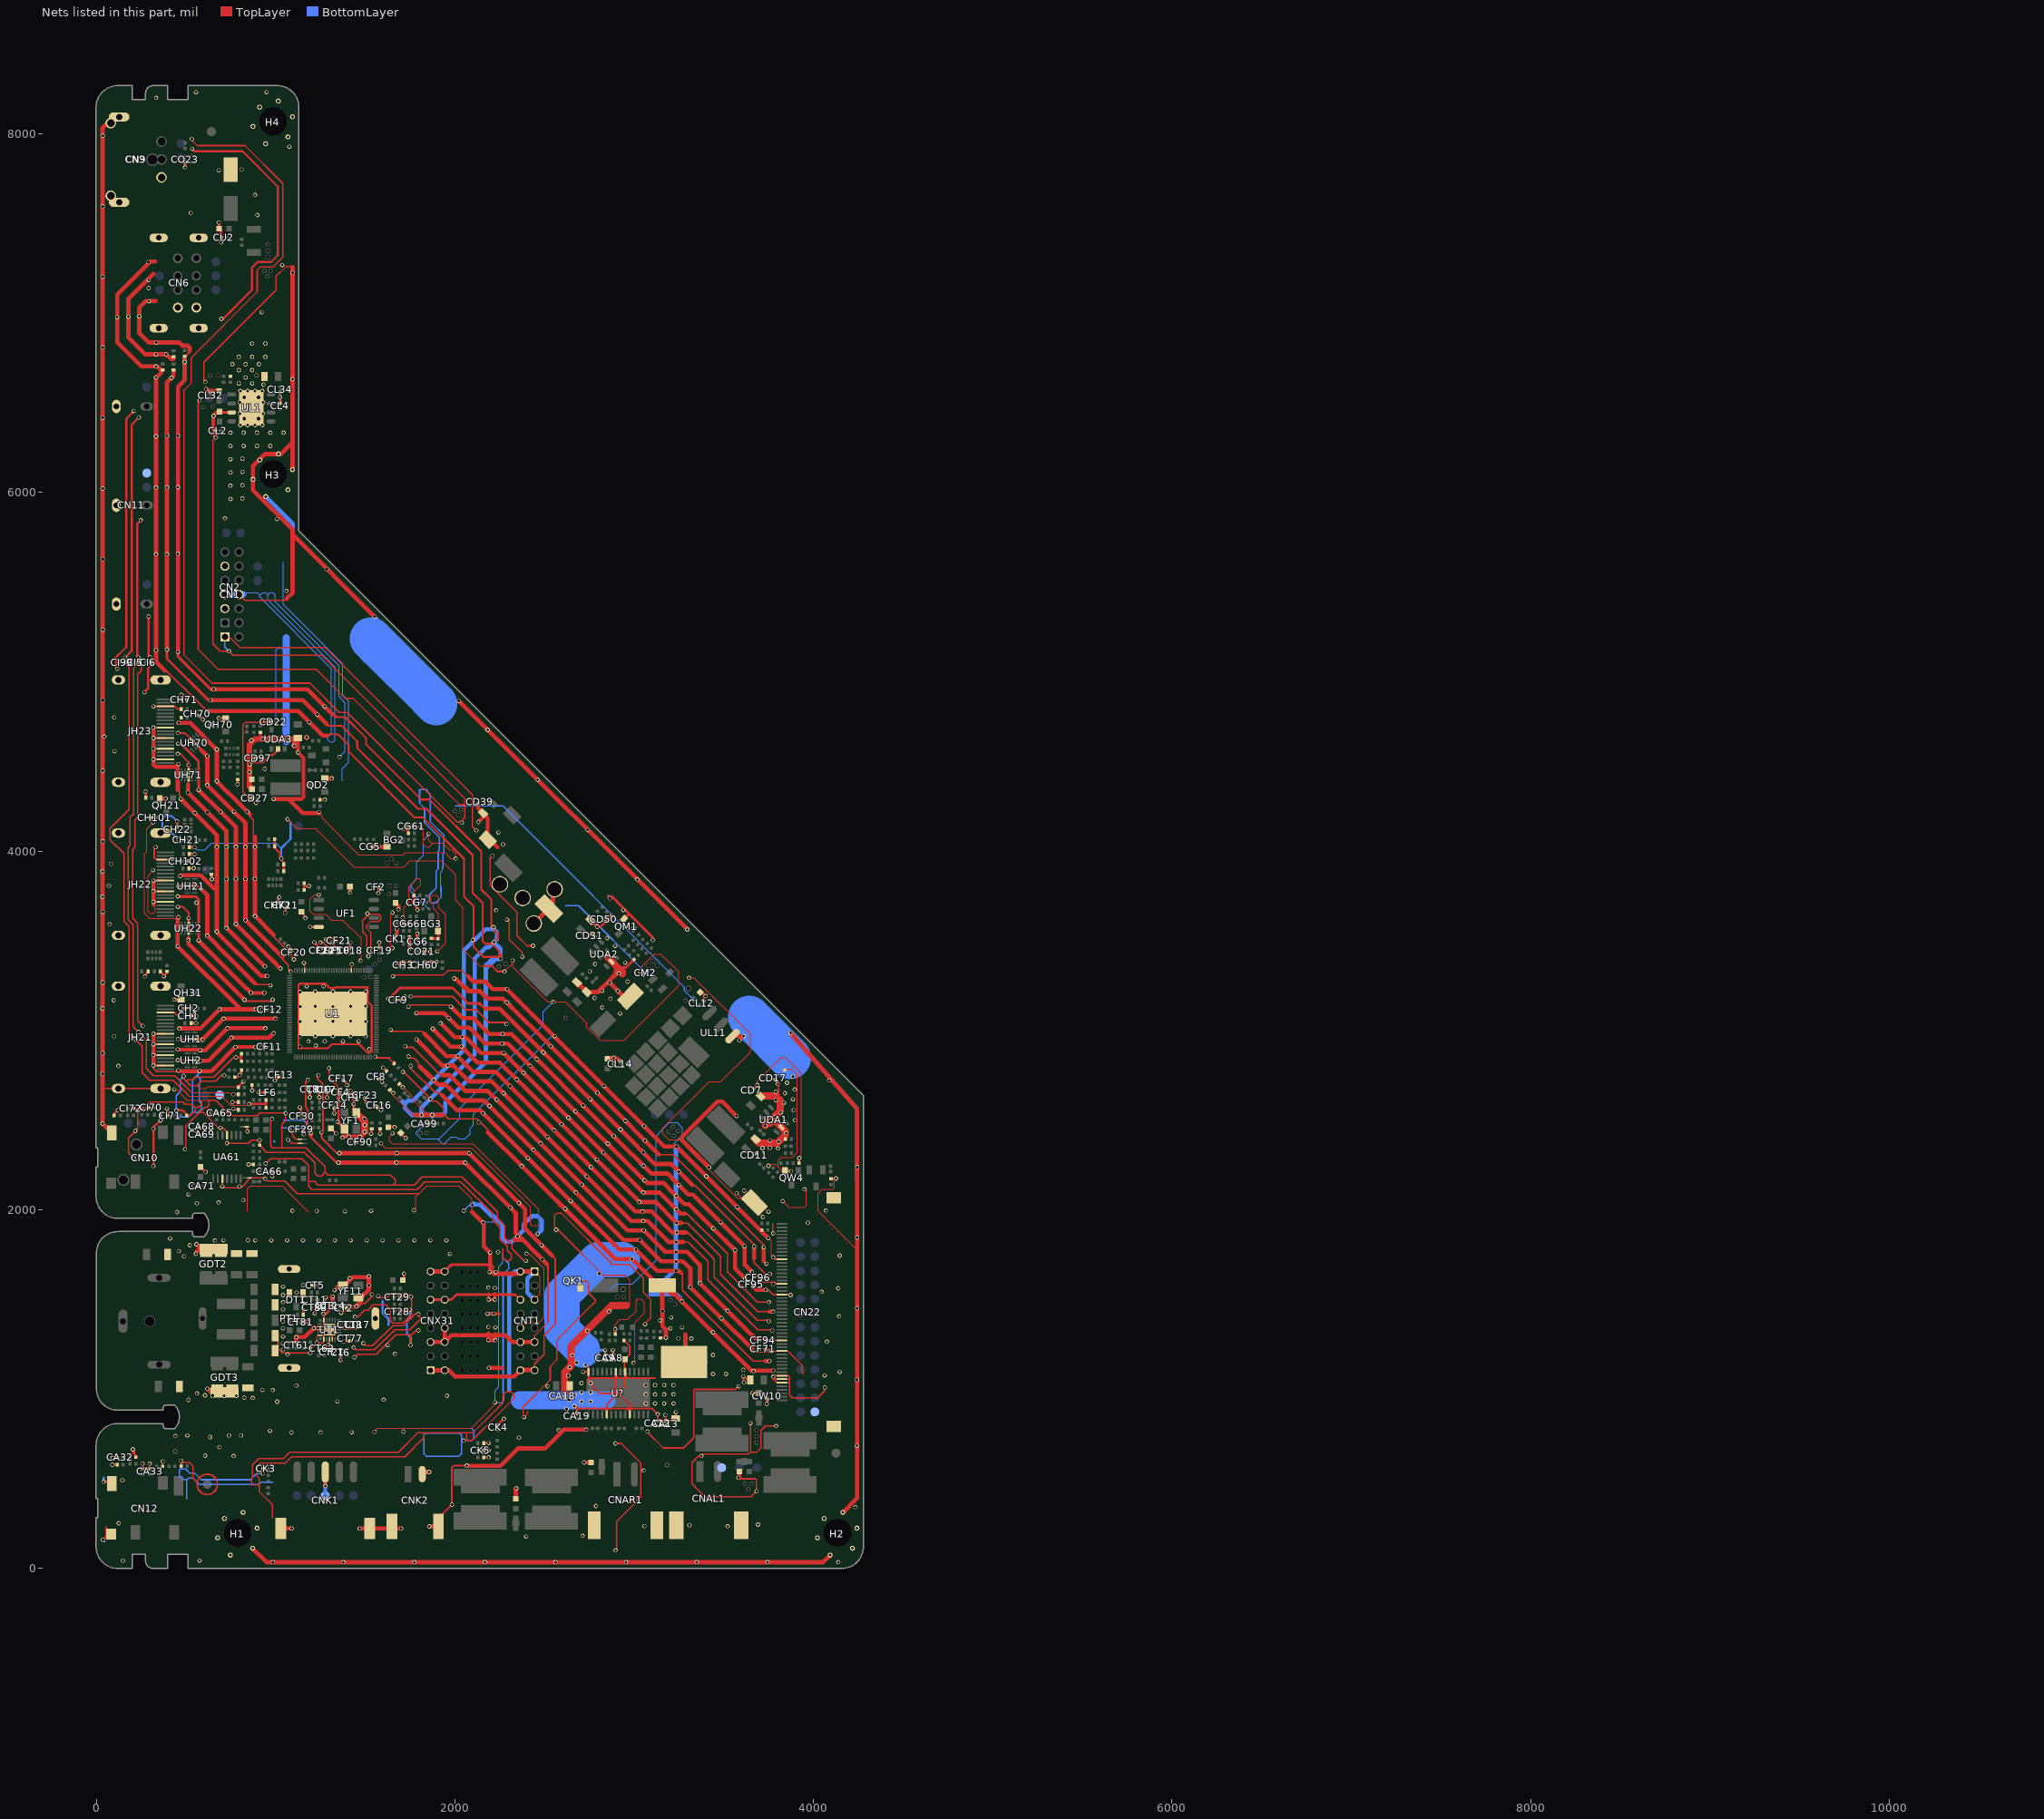
[diagram p0: the nets of this part, all layers, seen from the top]
# Altium PCB MISC105950.PcbDoc (part 8 of 15)
Units mil, origin at the board's own origin, x right, y up, seen from the top; angles counter-clockwise.
Board outline 4280.62 x 8272.76 mil, 2 copper layers (TopLayer, BottomLayer), stack 61.855 mil thick; 541 components, 268 nets, 2324 pads, 1157 vias.

## Via types
v1: diameter 23.62, hole 15.75, TopLayer to BottomLayer, tented both sides, 1087 vias
v2: diameter 23.62, hole 15.75, TopLayer to BottomLayer, 51 vias
v3: diameter 27.56, hole 19.68, TopLayer to BottomLayer, 15 vias
v4: diameter 31.5, hole 19.68, TopLayer to BottomLayer, tented both sides, 4 vias

## Nets (pads, with @x,y where several pads share a name; then routed paths per layer and width w, separated by ;. In a path a pad name is that pad's centre, name@x,y a point inside that pad or via, vN(x,y) a via of type N, cw(c..) or ccw(c..) an arc to the next point about the centre after c; other vN are vias at no path point) (continued)
GND: (continued)
  TopLayer w8: 41.8,2675.2 JH21.23@121.65,2675.2 JH21.22@356.3,2675.2 ; DA53.A@256.5,555.73 v2(256.5,582.5) ; CA33.2@297,555.24 v2(297,582) ; v2(369,595) 369.23,594.77 RA56.1@369.23,567 ; v1(432,2671) 443.41,2671 501.41,2613 ; DA51.A@471.27,565.23 DA51.A@471.27,568.5 471.27,597.27 v2(471.5,597.5) ; v2@471.27,588 471.59,588.33 495.5,588.33 ; v1@486,2743 v1(486,2743.5) ; 488,5163.35 488,5181.5 ; 491.09,588.33 495.5,588.33 ; v1(532,7972.38) 532,7963.5 534.61,7960.89 536.3,7960.89 561.69,7935.5 828.01,7935.5 1039.5,7724.01 1039.5,7312.78 984.72,7258 979.23,7258 979.12,7258.11 961.88,7258.11 961.77,7258 945.23,7258 ; 559.5,478.5 538,500 538,568 517.67,588.33 495.5,588.33 ; v1(574,6514) 567,6507 567,6486.5 ; v1@575,6514 575,6513 567,6505 567,6486.5 ; 575.25,2542.07 593.65,2542.07 679.71,2456 v1(691,2456) ; v1(606,6617.5) 599,6624.5 599,6726.95 1001.5,7129.45 1001.5,7206.88 1055,7260.38 1090.97,7260.38 ; v1(610.5,6578) 628.5,6560 CL32.2@635.43,6560 642.5,6567.07 CL31.2@683.93,6567.07 ; 648.5,6356.77 CL2.1@658,6347.27 ; 658.95,5145.42 649,5155.37 ; v1(665.5,6307) 649,6290.5 649,5155.37 ; 675,4936.5 692,4936.5 ; 712.09,5014.5 741.5,5014.5 ; CN1.1@715.6,5195.1 739.9,5195.1 799.5,5135.5 1275.66,5135.5 2097.5,4313.66 2097.5,4136 v1@2121.27,4112.23 ; CN2.6@794.34,5431.32 826.17,5399.5 1048,5399.5 1068.5,5420 ; 816.65,4705.7 829.64,4718.69 930.69,4718.69 v1(941,4729) ; 816.65,4705.9 816.65,4330.04 851.19,4295.5 CD27.1@865.43,4295.5 ; 816.65,4774.65 822.5,4780.5 ; 906.5,462.5 877.5,462.5 864.69,475.31 864.69,482 864.69,496.12 869.5,500.93 869.5,575.48 904.73,610.71 933,610.71 1042.33,610.71 1069.81,638.19 1078,646.38 1683.76,646.38 1792.73,755.35 2066,755.35 ; CK3.2@928.26,554.5 928.26,526.74 v2(928.5,526.5) ; 945.22,7258.01 914.01,7258.01 896,7240 896,7120.12 528.5,6752.62 528.5,6612 488,6571.5 488,5181.5 ; 980.5,279.5 980.5,335.5 ; 980.5,319 980.5,353 906.5,427 906.5,501.5 895.5,512.5 895.5,564.71 915.5,584.71 953,584.71 1053.1,584.71 1078.69,610.31 ; CT41.1@1012.06,1223.5 1035.56,1200 v1(1192.5,1200) ; 1071.69,603.31 1078.69,610.31 ; v1(1153,1442) v1@1153.23,1441.77 ; v1(1157,3377) 1160.04,3373.96 1160.04,3348 ; U1.124@1160.04,3334.04 1160.04,3348 ; 1160.04,3364.2 1160.04,3348 ; v1@1160.04,3367.05 1160.04,3348 ; 1172,5014.5 1163.5,5014.5 ; v1@1184.19,1191.68 v1(1192.5,1200) ; v1@1220.42,1330 v1(1212.89,1337.53) v1@1221.1,1345.75 ; 1229,1281.53 v1(1229,1256.5) ; 1260.78,1256.5 v1(1229,1256.5) ; UT1.EPAD@1283.75,1345.75 UT1.EPAD@1299.5,1330 ; v2(1294.25,1244.78) 1294.25,1240.97 CT21.1@1313,1222.23 ; U1.105@1421.85,3334.04 1421.85,3366.85 v1(1423.5,3368.5) ; v1@1470.98,3387.23 v1(1472.12,3388.38) ; v1(1511,3651) 1514.69,3647.31 1529,3647.31 ; v1(1516,3413.5) 1514.26,3411.76 1507.81,3418.21 1507.81,3526.4 1485.06,3549.15 1485.06,3612.12 1520.25,3647.31 1529,3647.31 ; v1(1539,3445.5) 1530.81,3453.69 1530.81,3545.13 1508.06,3567.88 1508.06,3585.12 1528.63,3605.69 1572.92,3605.69 1585.11,3617.88 1585.11,3635.12 1572.92,3647.31 1529,3647.31 ; v1(1653.25,3301.19) v1@1653.25,3307.81 ; v1@1654.44,3309 1654.44,3308.9 1717.5,3308.9 ; 1690.14,3309 1690.24,3308.9 1717.5,3308.9 ; 1831.5,755.35 1825.14,748.98 1825.14,726.21 1719.31,620.38 1088.77,620.38 1078.69,610.31 ; 1909.5,2527.31 1917.5,2519.31 ; v1@2038,4157.5 v1(2038,4158.5) ; v1(2048.58,711.19) 2075.38,711.19 ; 2054.5,4258.5 2024.5,4258.5 1948.18,4334.82 1430.13,4852.87 1384.92,4852.87 1223.29,5014.5 1163.5,5014.5 ; 2089.95,3284.05 2040,3334 1961.3,3334 1936.3,3309 1728.86,3309 1728.76,3308.9 1717.5,3308.9 ; CD96.1@2140.67,4213.05 2174.29,4179.42 ; v1(2208,3973.5) 2195.64,3961.14 2195.64,3808.36 2345.5,3658.5 2345.5,3527.85 2401.85,3471.5 v1(2434.5,3471.5) ; 2220.5,874.74 2207.63,861.87 ; v1(2229,3669.5) v1@2239,3669.5 ; 2256.69,910.93 2266.81,921.05 ; 2262.31,879.78 2244.52,861.98 ; 2266.81,930.69 2266.81,963.81 ; v1(2288.5,3617.5) 2288.5,3626 2290,3627.5 2302,3615.5 2302,3506.5 2374.87,3433.63 v1(2374.87,3410.13) ; v1@2379.9,840.7 2379.9,898.37 2530.86,1049.34 2530.86,1124.63 2566.86,1160.63 2566.86,1270.96 2740.2,1444.3 ; v1(2385,841) 2404,860 2404,873 ; 2556.19,1968.12 2568.38,1980.31 ; v1(2563.62,1886.98) 2574.67,1886.98 2600.83,1860.83 ; v1(2699,1600) 2735.5,1600 2744.5,1591 2744.5,1534.5 2782.4,1496.6 2782.4,1486.5 2740.2,1444.3 ; 2745.45,1449.55 2740.2,1444.3 ; 2750.85,1454.94 2740.2,1444.3 ; v1(2894.5,695) 2926.38,695 3035.5,585.88 3035.5,393.5 2902.5,260.5 2902.5,106 v1(2895,98.5) ; 2948.67,1632 2829.65,1632 2600.83,1860.83 ; v1(3060,1360) 3058,1362 3058,1363 3091.45,1396.45 3091.45,1497.78 3050,1539.24 3050,1616.93 2973.93,1693 2878.9,1693 2591.59,1980.31 2568.38,1980.31 ; v1@3071.5,759 3160.83,669.67 3196,669.67 ; RA1.2@3145.5,1284.27 v1(3176.23,1284.27) ; 3165.33,669.67 3196,669.67 ; 3301.5,697 3274.17,669.67 3196,669.67 ; 3337.6,603.5 3359.1,625 ; v1(3374.5,625) 3359.1,625 ; 3386.5,635.5 3376,625 3376,631 3380.5,635.5 3636.66,635.5 ; 3468.5,635.5 3636.66,635.5 ; v1(3580.19,503.94) 3586.63,497.5 3676.5,497.5 3681.5,492.5 v1(3681.5,428) 3650.5,397 3395,397 3322,470 3322,587.9 3359.1,625 ; 3647.5,644.5 v1(3647.5,808) ; v1(3763.2,1210.82) 3782,1210.82 ; v1@3768.62,1210.82 3782,1210.82 ; 3772.5,1923.5 3772.5,1869.76 v1(3775.11,1867.15) ; v1@3781.5,2617.5 3805.5,2641.5 3805.5,2702.5 CD17.2@3785.33,2722.67 3785.33,2715.17 v1(3800.5,2700) ; v1(3791.5,792) 3732.31,792 3707,766.69 3707,670.12 3681.86,644.98 3646.14,644.98 3636.66,635.5 ; 3945,1085 3934,1096 3934,1132.65 3863.02,1203.63 3862.69,1203.63 3855.51,1210.82 CN22.15@3823.43,1210.82 3782,1210.82 ; 488,5181.5 488,5093.29 644.79,4936.5 692,4936.5 ; 567,6486.5 567,5124.6 677.1,5014.5 741.5,5014.5 ; 649,5155.37 689.98,5114.39 v1(739.14,5114.39) 761.03,5092.5 1255.59,5092.5 2054.5,4293.59 2054.5,4186 2030.5,4162 2010.69,4162 1398.69,4774 1353,4774 1190.5,4936.5 692,4936.5 ; 741.5,5014.5 1163.5,5014.5 ; v1(1192.5,1200) LT4.1@1192.5,1226.77 1199.27,1226.77 v1(1229,1256.5) ; 2066,755.35 2101.11,755.35 2207.63,861.87 ; 2066,755.35 2063.19,752.54 2063.19,723.38 2075.38,711.19 ; 2075.38,711.19 2093.72,711.19 2244.52,861.98 ; 2207.63,861.87 2266.81,921.05 ; 2244.52,861.98 2330.52,947.98 2330.52,964.98 2313.5,982 2285,982 2266.81,963.81 ; 2266.81,921.05 2266.81,963.81 ; 2568.38,1980.31 2555.81,1967.74 2555.81,1905.84 2600.83,1860.83
  TopLayer w9: v1@3775.92,1733.23 3786.52,1722.63 CN22.41@3823.43,1722.63
  TopLayer w10: v1(317,2803) 317.15,2803.15 JH21.2@384.16,2803.15 ; v1(317,2862) 317.21,2862.21 JH21.5@384.16,2862.21 ; v1(317,2921.5) 317.24,2921.26 JH21.8@384.16,2921.26 ; v1(317,2980.5) 317.18,2980.32 JH21.11@384.16,2980.32 ; v1@317,3716.33 v1@317.21,3716.54 ; v1(317,3716.5) 317.04,3716.54 JH22.5@384.16,3716.54 v1@317.94,3716.54 ; v1(317,3775.83) 317.24,3775.59 317.94,3775.59 JH22.8@384.16,3775.59 ; v1(317,3834.83) 317.18,3834.65 JH22.11@384.16,3834.65 ; v1(317,4511.66) 317.15,4511.81 JH23.2@384.16,4511.81 ; v1(317,4570.66) 317.21,4570.87 JH23.5@384.16,4570.87 ; v1(317,4630.16) 317.24,4629.92 JH23.8@384.16,4629.92 ; v1(317,4689.16) 317.18,4688.98 JH23.11@384.16,4688.98 ; v1(317,4807) 317.09,4807.09 JH23.17@384.16,4807.09 436,4807.09 451.59,4791.5 DH72.A@472.77,4791.5 ; v1(330,4021.78) 321,4012.78 321,3964.5 332.74,3952.76 JH22.17@384.16,3952.76 ; 332,5060.49 335.54,5060.49 615.53,4780.5 v1(622.51,4780.5) ; JH21.17@384.16,3098.43 435.07,3098.43 v1(462.5,3071) ; v1@451.62,3686.71 451.62,3686.78 v1(452.95,3688.11) 482.39,3688.11 512.98,3657.52 v1@512.98,3613.5 ; v1@451.62,4541.04 451.62,4541.12 v1(452.95,4542.44) 466.06,4542.44 512.98,4495.52 UH71.GND@512.98,4444.3 ; v1(452.95,2833.78) 451.62,2832.45 451.62,2832.38 UH2.GND@547.47,2832.38 ; v1(454.5,2950.5) 454.62,2950.38 524.5,2950.38 ; v1@454.62,4659.04 v1(454.5,4659.16) 492.54,4659.16 UH70.GND@532.22,4619.48 ; v1(455.71,3804.71) 522.5,3804.71 ; v1(469.09,3123.27) 469.36,3123 CH2.2@495.76,3123 ; UH21.GND@506.53,3804.71 522.5,3804.71 ; UH22.GND@512.98,3549.03 v1@512.98,3613.5 ; UH22.GND@512.98,3589.97 v1@512.98,3613.5 ; 544.93,4606.78 580.72,4570.99 ; UH1.GND@547.47,2950.38 524.5,2950.38 ; 575.11,2950.38 524.5,2950.38 ; v1@580.22,3791.06 566.57,3804.71 522.5,3804.71 ; v1@640,3840 DH4.A@640,3866.77 ; v1(643,2539.5) CA65.2@671.26,2539.5 ; v1(691,2456) 704.5,2456 727.18,2433.32 UA61.4@727.18,2414.61 ; v1(758,2598) 759,2599 DI2.A@790.27,2599 ; v1(763,2562) 768.5,2556.5 DI33.A@789.77,2556.5 ; v1(824.82,3170.5) 831.82,3163.5 975.65,3163.5 v1(982.47,3170.31) ; RA64.JP_2K@837.76,2461.54 841,2458.3 v1(841,2436.5) ; CT41.1@1012.06,1223.5 CT42.1@1012.06,1309.37 ; v1(1178,2723) 1168,2713 1168,2569.59 1176.5,2561.09 1176.5,2447 v1(1194.5,2429) ; 1194.5,2405.96 1338.96,2261.5 v1(1348.86,2261.5) ; v1(1237.22,2748.94) 1233.5,2745.22 1233.5,2729 1263.84,2698.66 1263.84,2440.62 1254.84,2431.62 v1(1254.84,2430.47) 1254.84,2400.77 1341.11,2314.5 1370.81,2314.5 v1@1360.91,2314.5 ; CT10.2@1241,2652.76 1241,2627.72 v1(1242.62,2626.09) ; 1268,1406.52 1295.84,1434.36 1295.84,1473.66 1289.77,1479.73 CT3.1@1276,1479.73 ; v1(1554.5,2852.5) 1561.5,2845.5 1602.5,2845.5 ; v1(1598.61,2791.69) 1598.61,2791.39 DU31.A@1617.73,2772.27 ; 1636.15,2845.5 1602.5,2845.5 ; DU33.A@1636.33,2668.17 1655.16,2649.34 v1(1655.22,2649.34) ; DU32.A@1660.67,2814.33 1629.5,2845.5 1602.5,2845.5 ; DU34.A@1688.83,2700.67 1707.29,2682.21 v1(1708.09,2682.21) ; v1(1721.5,2910.5) 1728.44,2903.56 1765.14,2903.56 1919.02,2749.68 1928.92,2749.68 ; v1(1753,3189) 1787,3189 ; v1@1761.5,3189 1787,3189 ; CNK2.4@1907.13,277.89 v1(1982.86,353.62) 1982.86,462.5 ; 1982.86,441.36 1982.86,462.5 ; 2038.05,3261 2043.52,3255.52 2039.98,3255.52 ; 2066.5,3307.5 2103,3271 ; 2078.71,575.71 2073,570 1992,570 1982.86,560.86 1982.86,462.5 ; v1@2292,3040 2289,3043 2191.19,3043 2120.51,3113.68 2059.89,3113.68 1984.57,3189 1787,3189 ; v1(2486.69,1721.55) 2486.69,1721.82 2473,1735.5 2473,1725.61 2519,1679.61 2519,1663.5 ; 2519,1374.42 2519,1663.5 ; 2519,1699.41 2519,1663.5 ; 2529.78,1753.68 2558,1725.46 2558,1362.5 ; v1(2636,937.5) 2636,937.73 CA18.1@2615.23,958.5 2639.53,982.8 CA2.1@2639.53,1017 ; 2672.98,889.93 3098.57,889.93 v1(3130.5,858) CA12.1@3130.5,823.23 3221.2,823.23 CA1.1@3231,833.03 v1(3231,869) ; CA19.1@2680,865.23 2680,899.5 ; v1(2714.5,1094.5) U?.14@2743.87,1094.5 ; v1(2727.87,1132.13) 2743.87,1116.14 U?.14@2743.87,1094.5 ; 2830.23,889.93 U?.19@2846.23,873.93 ; U?.19@2846.23,854.34 2846.23,910.44 2910.2,974.42 ; U?.19@2846.23,877.14 2859.02,889.93 ; 2884.61,1058.91 2897.41,1071.7 ; 2897.41,987.22 U?.8@2897.41,1094.5 ; U?.8@2897.41,1074.91 2913.41,1058.91 ; 2935.8,1058.91 2948.59,1071.7 U?.6@2948.59,1094.5 ; RA9.1@2942.77,1270 2942.95,1270 2972.75,1240.2 2972.75,1190.44 CA7.1@2957.61,1175.3 ; U?.6@2947,1096.09 CA7.1@2947,1164.69 ; 2958.18,889.93 U?.24@2974.18,873.93 ; 2964.59,1058.91 2948.59,1074.91 U?.6@2948.59,1094.5 ; U?.24@2974.18,854.34 2974.18,910.44 2910.2,974.42 ; U?.24@2974.18,877.14 2986.98,889.93 ; v1@3071.5,759 3071.5,759.5 v1(3073.5,761.5) ; 3116.09,1058.91 2757.46,1058.91 2743.87,1072.5 U?.14@2743.87,1094.5 ; CA13.1@3173,822.89 v1(3173,853.5) ; 3275.17,670.67 3331.86,727.36 3331.86,811 ; 3331.86,769.36 3331.86,811 ; v1@3583,1016 3564.29,997.29 3337.72,997.29 3331.86,991.43 3331.86,811 ; v1(3611.65,1035.18) 3608,1038.83 v1(3608,1069) 3612,1069 3632,1049 CW9.1@3647.47,1049 ; v1(3659,975) v1@3659.31,975.31 ; U?.14@2743.87,1094.5 2743.87,1037.13 2806.58,974.42 2910.2,974.42 ; 2910.2,974.42 2948.59,1012.81 U?.6@2948.59,1094.5
  TopLayer w11: 1255.88,4650.5 1347.54,4650.5 1406.5,4591.54 1406.5,4554.99 1774.49,4187 1820.53,4187 2050.5,3957.03 2050.5,3745.5 2103.15,3692.85 2103.15,3580 ; 1284.96,4707.69 1294.15,4698.5 1340.5,4698.5 ; 1312,4698.5 1340.5,4698.5 ; CF3.1@1413.81,3802 1414,3801.81 v1(1414,3768) ; CG7.1@1767.27,3714 CG7.1@1770,3716.73 ; v1(2099,3504) 2103.15,3508.15 2103.15,3580 ; 2165.42,3358.5 2206.17,3358.5 2236.67,3328 v1(2275,3328) ; v1(2214.67,3575.26) 2213.95,3575.26 2201.72,3587.5 ; 2246.31,3409.5 2158.5,3409.5 2103.15,3464.85 2103.15,3580 ; 2246.31,3414.81 2246.31,3441.69 2215.88,3472.12 v1@2215.88,3490.88 ; 1340.5,4698.5 1367.42,4698.5 1454.5,4611.42 1454.5,4574.87 1793.87,4235.5 1840.13,4235.5 2098.5,3977.13 2098.5,3765.39 2153.72,3710.17 2153.72,3516.51 2153.72,3498.03 2169.24,3482.5 2207.5,3482.5 v1@2215.88,3490.88 ; 1341.61,4746.5 1324.4,4763.71 1315.21,4763.71 1332.42,4746.5 1341.61,4746.5 ; 1341.61,4746.5 1387.3,4746.5 1502.59,4631.21 1502.59,4595.81 1810.75,4287.65 1856.12,4287.65 2146.5,3997.27 2146.5,3785.27 2201.72,3730.05 2201.72,3587.5 ; 2201.72,3587.5 2201.72,3576.78 2238.5,3540 2238.5,3513.5 v1@2215.88,3490.88
  TopLayer w12: v1(35,157.5) 53,175.5 53,226 ; v1(39,480.5) 74.62,480.5 CN12.2@84.65,470.47 ; v2(87.5,576.5) DA52.A@114.27,576.5 ; v2(88,615) 119.65,615 CA32.2@121.65,617 ; DI34.A@98.77,2524.5 98.77,2534.27 v1(118.5,2554) ; v1(115.5,5018) 115.5,5019 106.9,5027.6 106.9,5079.62 165.5,5138.21 165.5,6411.5 v1@208.25,6454.25 ; CI99.1@160.23,5052 160.23,5079.77 v1(160,5080) 195.5,5115.5 195.5,6377.88 v1@236.61,6418.99 ; RA55.1@220.23,618 RA55.1@220.23,625.97 ; CI5.1@233.73,5052 233.73,5079.77 v1(233.5,5080) 226,5087.5 226,5825.5 v1(246.5,5846) ; v1(267,4885.5) v1@267,4886.5 ; v1(269.5,3300) 269.5,3307 286.23,3323.73 DH81.A@286.23,3328.5 ; v1(272,4332) 274.04,4329.96 DH21.A@274.04,4297.5 ; 282.31,4901.81 v1@267,4886.5 ; 284,4903.5 v1@267,4886.5 ; v1(290,5308.38) 290,5088.5 v1(297.5,5081) 305.23,5073.27 CI6.1@305.23,5052 ; CH101.1@305.93,4187.5 305.93,4169.07 v1(315.5,4159.5) ; CI6.1@307.23,5052 307.23,5039.23 287.77,5019.77 287.77,4907.27 v1@267,4886.5 ; v1(317,2242.5) v1(317,2450) 317,2458.54 355.46,2497 v1(357,2497) ; v1@355.23,2498.77 DI23.A@355.23,2528.5 ; DH2.A@356.73,3328.5 375.5,3309.73 v1(375.5,3301) 392.5,3318 DH3.A@392.5,3327.77 ; v1(392.5,2562) 394.27,2560.23 CI71.1@394.27,2524.5 ; v1(433.5,3171) QH31.E@471,3171 ; v1(445.5,2553) 481,2553 DI24.A@502.46,2531.54 ; CH22.2@449.5,4138.24 v1(449.5,4165.5) ; v1(456.94,4063.36) 458.2,4062.1 CH21.2@483.61,4062.1 ; v1(472,4871.5) 472.5,4871 487.5,4871 505.23,4853.27 CH71.2@505.23,4843.5 ; 488,2546 DI24.A@502.46,2531.54 ; DU1.A@491,6759.65 495.93,6759.65 516.5,6780.21 516.5,6811.34 508.87,6818.97 ; DI24.A@502.46,2524.5 DI24.A@502.46,2531.54 ; DH22.A@518.79,3984.1 543.48,3984.1 v1(545.46,3982.12) ; DH23.A@518.79,4022.1 519.16,4021.74 v1(545.46,4021.74) ; DH1.A@526.96,3040 v1(554,3040) ; CH1.2@529.24,3081 531.62,3078.62 v1(555.91,3078.62) ; v1(532.5,7916.88) 545.88,7903.5 814.76,7903.5 1011.5,7706.76 1011.5,7324.38 973.23,7286.11 899.11,7286.11 867,7254 867,7130.71 v1@702.89,6966.61 ; v1(541.5,2131.5) CA71.2@575.5,2131.5 ; CH70.2@568.47,4758.03 569.47,4758.03 v1(593,4734.5) ; CA69.2@568.93,2420 548.19,2440.74 v1(548.19,2440.95) CA68.2@568.93,2461.69 ; CA70.2@579.5,2237.69 607.31,2209.88 v1(608.37,2209.88) ; v1(682.5,4742) QH70.E@720,4742 ; RF19.2@771.73,2739.5 786,2739.5 ; v1(778.54,2848.54) 806.04,2848.54 ; v1(785.84,4372.36) 787.75,4374.27 RH75.2@787.75,4399.03 ; RI21.1@790.27,2682.5 790.27,2684.77 v1(819.5,2714) v1@811.27,2705.77 ; v1(798.5,2750.5) 797,2750.5 786,2739.5 ; RI36.1@806.04,2827.5 RI23.1@806.04,2869 ; RI25.1@808.04,2778.5 808.04,2761.54 786,2739.5 ; v1(847.76,2251.5) RA71.1@875.77,2251.5 ; v1(851.16,2588.84) 883,2588.84 ; v1@854.16,4494 926.71,4494 967.86,4535.14 983.99,4535.14 1012.5,4563.65 UDA3.2@1012.5,4569.37 ; 857,4517.5 CD97.2@884.04,4517.5 ; v1@862.66,2588.84 883,2588.84 ; CD27.1@865.43,4295.5 865.43,4284.09 881.67,4267.85 v1(889.89,4267.85) ; RF12.2@868.37,2693.4 868.37,2670.67 v1@870.5,2666.5 ; v1@904.5,2652.5 LF6.1@932,2652.5 ; v1(909,2387) 909.23,2386.77 RA69.1@909.23,2359.25 ; v1(919.5,2905.5) 921,2907 CF11.2@946.54,2907 ; v1(922,3117.5) 924,3115.5 CF12.1@948.77,3115.5 ; 928.59,4716.59 v1(941,4729) ; v1@933.5,4721.5 CD22.1@967.93,4721.5 ; v1@943,2254.5 v1(943,2256.5) ; RI16.2@946,2568 946,2588.5 ; RI14.2@946,2610 946,2588.5 ; CA66.1@979.89,2213.5 979.89,2185.61 v1(980,2185.5) ; DH73.A@993.5,4065.5 DH74.A@993.5,4027.5 993.5,4018.26 1024.04,3987.72 1024.04,3964.55 v1(1029.85,3958.74) 1029.85,3950.69 1044,3936.54 DH76.A@1044,3926 DH75.A@1044,3887.5 ; CH72.1@1011.5,3715.12 1011.5,3734 v1(1019.29,3741.79) ; CL4.2@1023.5,6499.74 v1@1023.5,6531.5 ; v1(1051.69,3655) 1053.5,3656.8 CK11.2@1053.5,3681.67 ; v1(1070,3467) 1087.84,3449.16 CF20.1@1087.84,3446.16 ; 1126.5,3060.76 1157.62,3091.88 U1.EPAD@1318.5,3091.88 ; v1(1134,2569.5) 1140,2563.5 1140,2541.46 CF30.2@1144.5,2536.96 ; CF5.1@1140,3658.69 1164.5,3634.19 v1(1164.5,3626.5) ; v1(1156,2419) 1156.24,2419.24 CF29.2@1156.24,2447 ; CD102.A@1157.73,3783 1157.73,3805 ; CD101.A@1157.73,3821 1157.73,3805 ; v1(1185,3805) 1157.73,3805 ; CT8.1@1189,2652.77 1190,2651.77 v1(1190,2626) ; v1(1192,3576.5) UF1.4@1239.5,3576.5 ; v1(1248.5,3490) 1261.5,3490 1290.43,3461.07 CF25.2@1299.5,3461.07 ; CT62.2@1273.24,1224.5 1277.78,1224.5 v2@1294.25,1240.97 ; v1(1280,3507) 1285.5,3512.5 1323.43,3512.5 CF21.2@1335.43,3500.5 ; v1(1285.5,2624.5) CF7.1@1285.5,2651.43 ; CF6.1@1307,2452.5 1334.81,2424.69 v1(1335.87,2424.69) ; v1(1308.76,3487.74) 1309.26,3487.74 1335.93,3461.07 CF10.1@1341.5,3461.07 ; v1(1326.5,2537) CF14.1@1326.5,2564.01 ; v1(1344.5,2489) 1381.3,2452.2 YF1.4@1382.57,2452.2 ; 1349.92,2511.88 1349.92,2564.5 ; 1349.92,2622.04 1349.92,2564.5 ; v1(1361,1160) 1361.5,1160.5 CT6.1@1361.5,1186.77 ; v1(1361.5,2612) CF4.1@1361.5,2638.93 ; v1(1378.23,1263.27) CT77.1@1412.5,1263.27 ; v1(1407.5,2406.83) 1407.83,2406.5 1429,2406.5 ; CF18.2@1414,3461.24 1414,3486 v1(1416,3488) ; v1(1425.5,2377) CF90.2@1452.26,2377 ; v1@1492.82,2505.32 v1(1494.57,2505.32) ; v1(1496.15,2471.5) v1(1496.15,2433.97) v1(1468.68,2406.5) 1429,2406.5 ; CF23.1@1497,2620.77 1497,2607.59 v1(1510.5,2594.1) ; v1(1531.45,2422.6) 1534.5,2425.65 DK2.A@1534.5,2449.27 ; CF16.1@1564.13,2569.63 1570.78,2569.63 v1(1587.01,2553.4) ; CF8.1@1573.33,2729.67 1591.4,2711.6 v1(1592.97,2711.6) ; CF19.2@1577,3455.84 v1(1577,3489.5) ; DK3.A@1581.5,2449.27 1581.5,2423.24 v1(1582.14,2422.6) ; CF58.1@1627.5,2448.52 CF58.1@1627.5,2458.69 1632.5,2463.69 1658.81,2463.69 v1(1663,2459.5) ; CT29.2@1693.74,1510.5 1705.32,1510.5 v1(1720.18,1525.35) ; CT28.1@1694.73,1431.5 1696.73,1433.5 1739.5,1433.5 v1(1747,1441) ; CF59.1@1696,2427 1724.35,2398.65 v1(1724.35,2398.31) ; v1(1707,3629) 1707,3600.27 CG66.1@1712.27,3595 ; CT80.1@1715.12,1605.5 v1(1715.12,1641.38) ; CO21.1@1827.73,3438.5 v1(1862.23,3438.5) ; CA99.1@1846.07,2478.5 v1(1873,2478.5) ; CK5.1@2152.84,656.5 v1(2186.5,656.5) ; DK4.A@2160.73,616.5 2186.5,616.5 v1(2187.5,617.5) ; DK70.A@2160.73,697 v1(2187.5,697) ; QK1.E@2699,1562.5 v1(2699,1600) ; v1(2836.26,1215.9) 2837.44,1214.72 CA9.1@2837.44,1189.23 ; v1(2879.88,1215.9) 2881.84,1213.94 CA8.1@2881.84,1189.23 ; v1(3031,3329) 3032.84,3329 CM2.1@3051.67,3310.17 ; CD7.2@3666.37,2675.87 v1(3685.5,2695) ; CF71.1@3733.24,1221.48 3737.34,1217.38 3756.64,1217.38 v1(3763.2,1210.82) ; QW4.E@3840.5,2216 3870.19,2216 v1(3874.06,2212.13) ; v1@3919.5,2286 RW14.2@3919.5,2259.5 3919.5,2286.3 v1(3920.35,2287.15) ; RA55.1@220.23,625.97 203,643.2 v2(203,662) 208.96,656.04 208.96,637.24 RA55.1@220.23,625.97 ; 883,2588.84 945.66,2588.84 946,2588.5 ; 1349.92,2564.5 1349.92,2484.85 YF1.4@1382.57,2452.2 ; YF1.4@1382.57,2452.2 1382.57,2436.93 1413,2406.5 1429,2406.5 ; 1126.5,2899.7 1126.7,2899.5 1289.61,2899.5 1312.11,2922 1465.2,2922 1512.7,2874.5 1524.65,2874.5 1525.19,2873.96 1535.88,2884.64 1535.88,3136.08 1511.92,3160.03 1511.92,3239.26 1333.02,3239.26 1328.95,3235.19 1300.87,3235.19 1276.8,3259.26 1133.44,3259.26 1126.5,3252.31 1126.5,2899.7
  TopLayer w15: CI72.1@200.34,2564 283.77,2564 CI70.1@288.27,2568.5 ; v1(393,5124) 393,5073.03 624.53,4841.5 v1(636,4841.5) ; v1(454,5110.28) 454,5085.57 472.53,5067.03 ; v1(455,4599.5) 457,4597.5 472.5,4597.5 568.35,4501.65 568.35,4465.86 568.98,4465.23 568.98,4423.38 568.98,4341.53 v1(569.16,4341.36) ; 463,5076.57 472.53,5067.03 ; v1(493,7815) CO23.1@493,7842.15 ; 528.17,3745.83 552.67,3745.83 569.16,3729.34 569.16,3538.5 ; v1(569.16,3501.11) 569.16,3538.5 ; 569.16,3515.37 569.16,3538.5 ; 637.07,4902.5 472.53,5067.03 ; 648.5,6356.77 648.5,6427.5 668,6447 UL1.3@753.95,6447 ; v1(683,7506.5) 683.19,7506.31 CU1.1@683.19,7472.88 ; v1(694.26,7394.76) CU2.2@694.26,7423.88 CU1.1@694.26,7461.8 ; 913,4626 RD88.1@913,4663.27 ; v1(994.5,2720.5) CF13.1@1014.67,2740.67 ; LT2.1@1153.23,1413 v1@1153.23,1441.77 ; v1(1214.68,3490.08) 1214.68,3488.32 1241.93,3461.07 CF24.1@1257,3461.07 ; v1(1216.5,1420.5) 1219.67,1423.67 1219.67,1436.34 1231.71,1448.38 CT11.1@1231.71,1496.4 ; CF17.1@1377.33,2719.67 1398,2699 v1(1398,2693.5) ; v1(1384.5,1338.5) CT17.2@1452.74,1338.5 ; v1(1416.5,2663) 1434.39,2645.11 CF1.1@1434.39,2625 ; YF1.2@1434.39,2553.93 CF1.1@1434.39,2625 ; v1(1434.39,2587.61) CF1.1@1434.39,2625 ; v1(1572,3765.5) 1574.73,3768.23 CF2.1@1574.73,3798 ; v1(1626.69,3176.31) 1626.69,3182.68 1638.78,3182.68 1692.1,3236 1800,3236 ; v1(1676.5,3360.5) 1697.23,3381.23 RH82.2@1749.5,3381.23 ; 1710.73,3181 CF9.1@1698.23,3168.5 1719,3189.27 v1(1719,3189.5) ; v1@1713.5,4121 1737.27,4121 ; CG61.1@1737.27,4138.5 1737.27,4121 ; RG8.1@1740.27,4100.5 1737.27,4103.5 1737.27,4121 ; RG9.1@1769.77,3752 1769.77,3703.23 1784,3689 ; v1(1790,3671) 1784,3677 1784,3689 ; v1@1792,3681 1784,3689 ; CH60.1@1828.5,3381.23 1828.73,3381 v1(1896.5,3381) ; CNX31.1@1863.21,1102.99 CNX31.2@1941.95,1102.99 ; CNX31.11@1863.21,1496.69 1979.69,1496.69 ; DO21.A@1867.5,3512.23 1904,3512.23 RO22.1@1904.5,3511.73 ; 1895,3236 1800,3236 ; RO22.1@1907,3514.23 v1(1907,3597.5) ; CNX31.16@1941.95,1654.17 1980.78,1693 2198,1693 2214,1677 ; 1964.5,1496.69 1979.69,1496.69 ; 1986.36,3236 2072.36,3150 2132.98,3150 ; 1986.9,3236 1800,3236 ; 2069,3305 2089.95,3284.05 ; 2140.22,3142.76 2132.98,3150 ; v1(2182,1418) 2247,1418 ; 2187.5,1531.5 v1(2187.5,1497.5) v1(2221.5,1497.5) 2221.5,1531.5 ; CK4.1@2240,801.23 2271.04,832.26 v1(2272.51,832.26) ; 2240.32,3125.18 2163.74,3125.18 2138.92,3150 2132.98,3150 ; CNT1.6@2364.47,1496.63 2336.1,1525 2008,1525 1979.69,1496.69 ; CD31.2@2760.83,3539.33 2761.67,3539.33 v1(2781,3520) ; v1(2792.78,3577.5) 2811.17,3577.5 CD50.2@2840.83,3607.17 2869.33,3635.66 RD53.2@2869.33,3637.67 ; CL13.1@2853,2837.81 2865.19,2850 v1@2882,2850 ; CL13.1@2853,2841.31 v1@2883.5,2841.31 ; v1@2856.5,3742 v1@2856.5,3744.5 ; 2858.5,3746.5 v1@2856.5,3744.5 ; UDA2.2@2874.5,3381.5 2906.5,3349.5 2953.5,3349.5 RD54.1@2998.17,3394.17 ; v1@2883.5,2819.93 v1@2883.5,2841.31 ; v1@2893.42,2841.31 v1@2883.5,2841.31 ; v1(2893.5,1333.5) 2893.67,1333.33 RA11.1@2893.67,1305.5 ; QM1.E@2942.27,3620.8 2968.55,3647.09 2974.09,3647.09 ; v1(3103,3503) 3103,3518.17 2974.09,3647.09 ; CL11.1@3363.17,3206.17 3382.51,3206.17 v1(3397.5,3191.17) 3387.83,3181.5 CL12.1@3387.83,3162.33 ; v1(3739.5,915.5) 3741.5,917.5 CW10.1@3741.5,942.27 ; v1@2856.5,3744.5 2876.67,3744.5 2974.09,3647.09 ; v1(2885,2847) 2897.34,2847 2914.61,2829.73 CL14.1@2921.5,2829.73 2904.23,2847 v1(2885,2847)
  TopLayer w16: 671,4906.5 675,4902.5